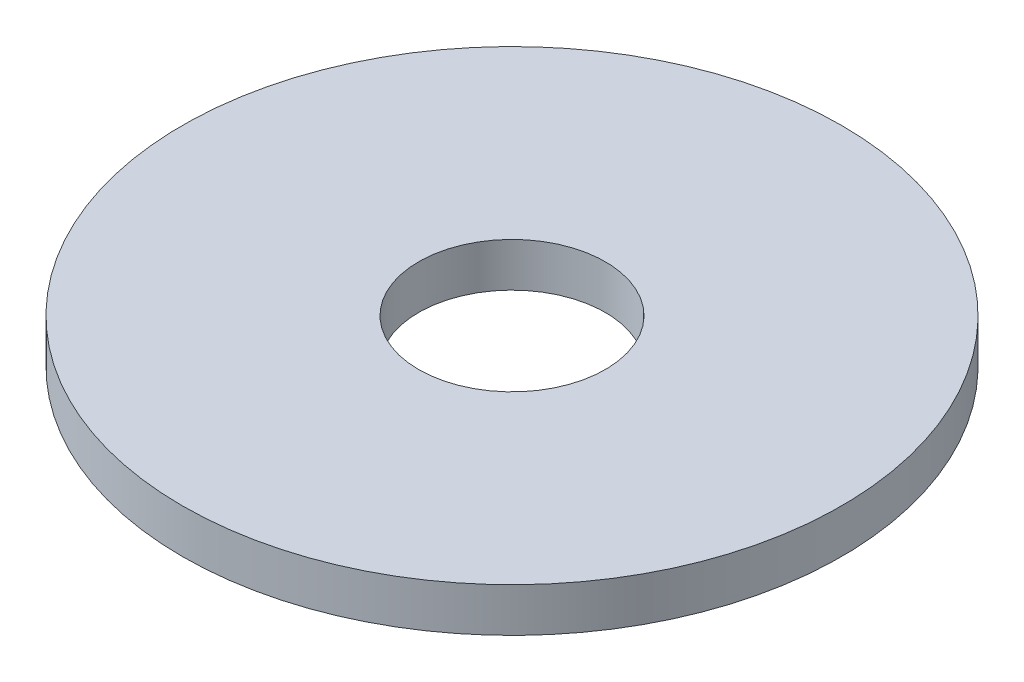
from build123d import *

# Parameters (mm, degrees)
SKETCH1_R      = 30
SKETCH1_R_2    = 8.5
EXTRUDE1_DEPTH = 2


with BuildPart() as part:
    # Sketch1 → Extrude1 (new, symmetric)
    with BuildSketch(Plane(origin=(0, 0, 0), x_dir=(1, 0, 0), z_dir=(0, 1, 0))):
        with Locations(Location((0, 0, 0), (0, 0, 270))):
            Circle(SKETCH1_R)
        with Locations(Location((0, 0, 0), (0, 0, 270))):
            Circle(SKETCH1_R_2, mode=Mode.SUBTRACT)
    extrude(amount=EXTRUDE1_DEPTH, both=True)


solid = part.part
